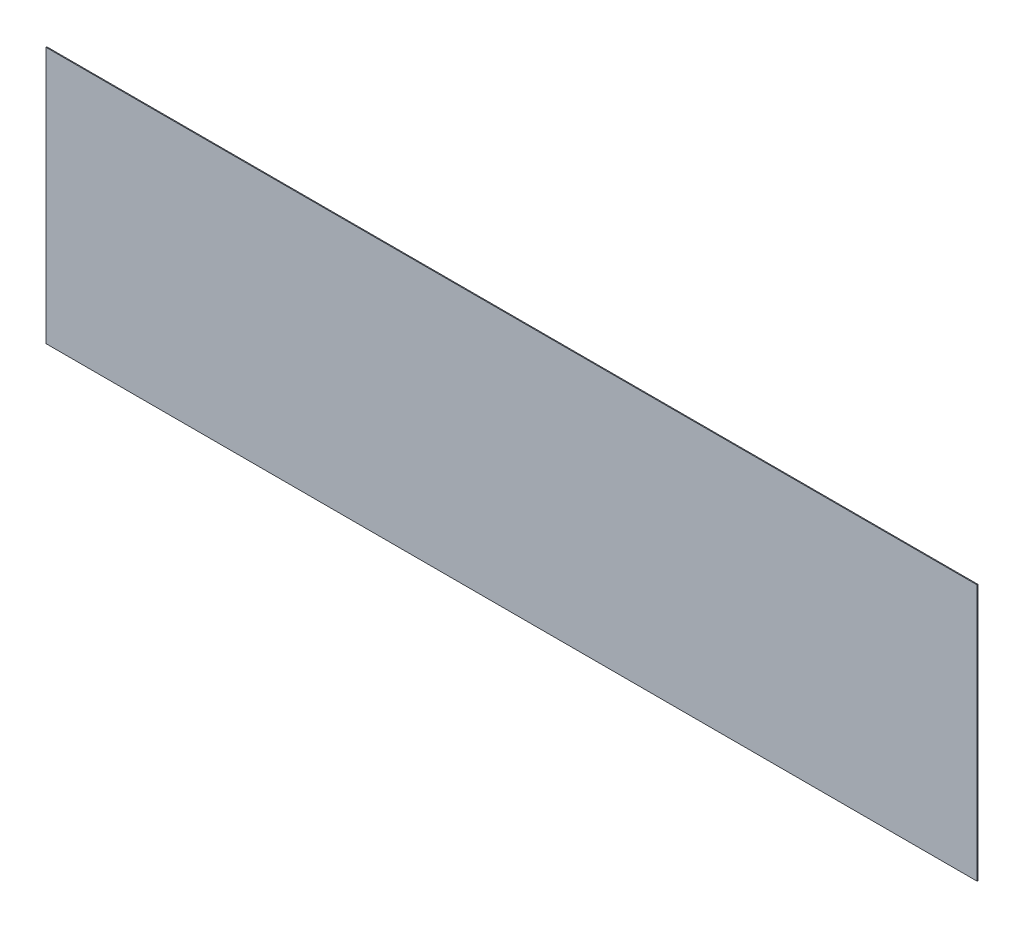
from build123d import *

# Parameters (mm, degrees)
SKETCH1_W           = 1560
SKETCH1_H           = 430
BOSS_EXTRUDE1_DEPTH = 1.5


with BuildPart() as part:
    # Sketch1 → Boss-Extrude1 (new body)
    with BuildSketch(Plane.XY):
        with Locations((780, 215)):
            Rectangle(SKETCH1_W, SKETCH1_H)
    extrude(amount=BOSS_EXTRUDE1_DEPTH)


solid = part.part
